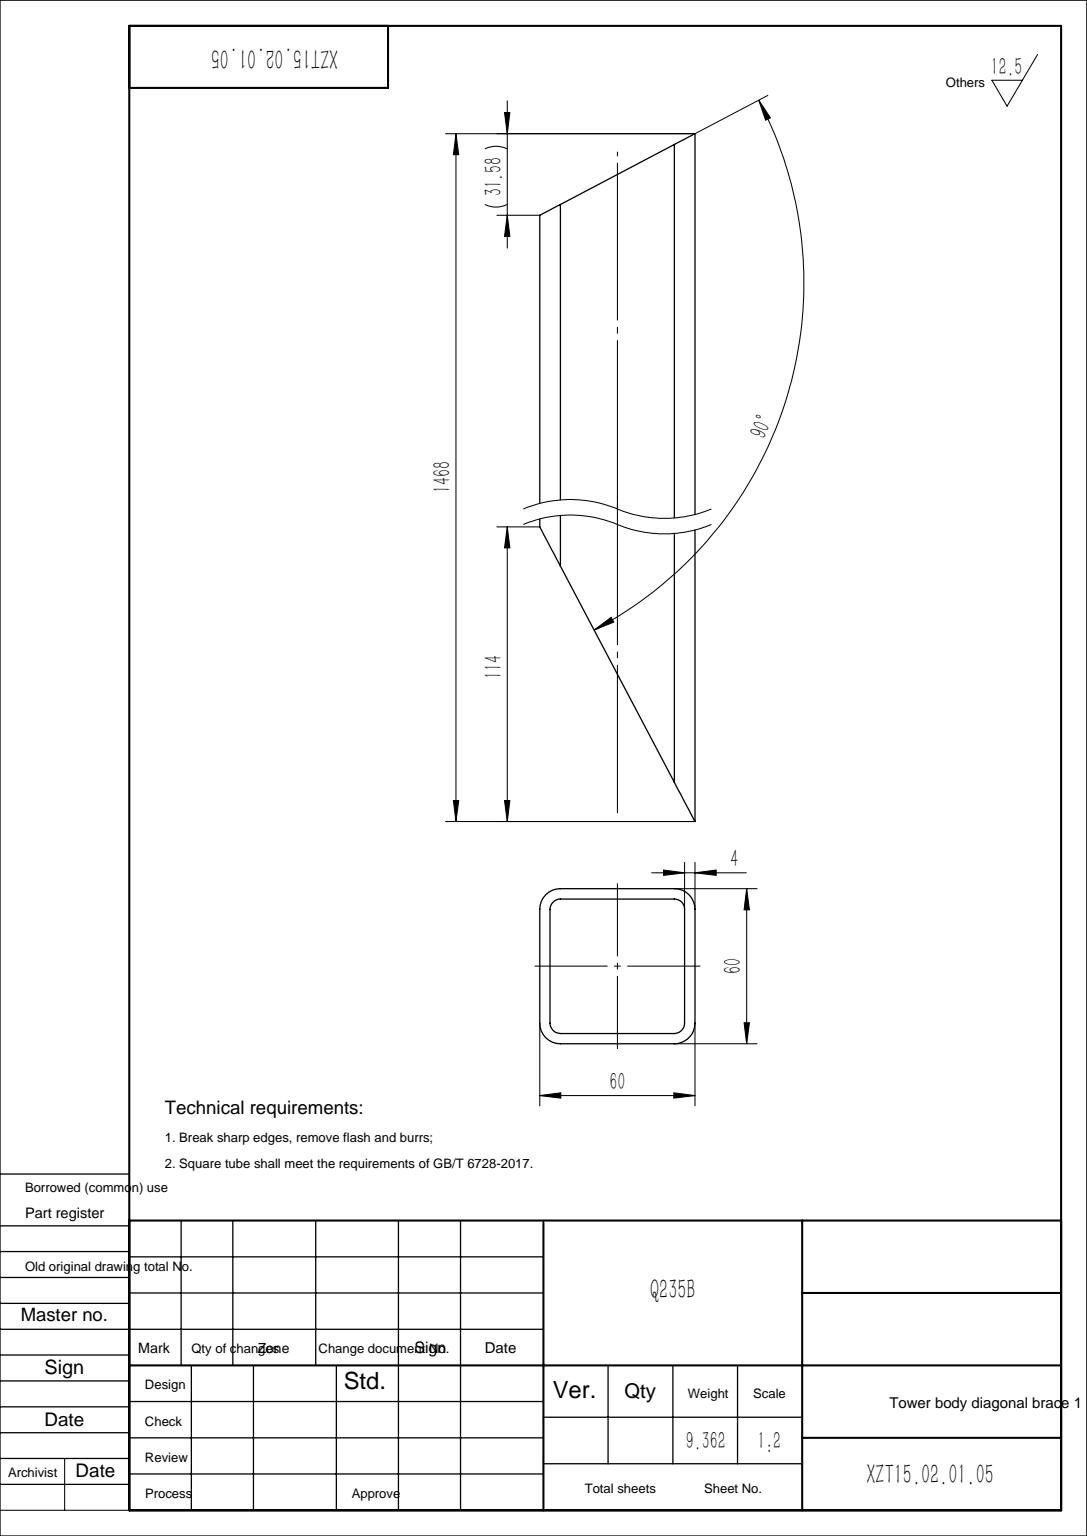
from build123d import *

# Parameters (mm, degrees)
GB_T_6728_2002_SQUARE_HOLLOW_SECTION_60_DEPTH = 1468
CUT_EXTRUDE1_DEPTH                            = 1470.531898259
CUT_EXTRUDE1_DEPTH_BACK                       = 1470.531898259


with BuildPart() as part:
    # Sketch1 → GB/T 6728-2002 square hollow section 60×60×4(1) (new body)
    with BuildSketch(Plane(origin=(0, 0, 0), x_dir=(-1, 0, 0), z_dir=(0, 1, 0))):
        with BuildLine():
            Line((-22, -30), (22, -30))
            ThreePointArc((22, -30), (27.656854249, -27.656854249), (30, -22))
            Line((30, -22), (30, 22))
            ThreePointArc((30, 22), (27.656854249, 27.656854249), (22, 30))
            Line((22, 30), (-22, 30))
            ThreePointArc((-22, 30), (-27.656854249, 27.656854249), (-30, 22))
            Line((-30, 22), (-30, -22))
            ThreePointArc((-30, -22), (-27.656854249, -27.656854249), (-22, -30))
        make_face()
        with BuildLine():
            Line((-22, -26), (22, -26))
            ThreePointArc((22, -26), (24.828427125, -24.828427125), (26, -22))
            Line((26, -22), (26, 22))
            ThreePointArc((26, 22), (24.828427125, 24.828427125), (22, 26))
            Line((22, 26), (-22, 26))
            ThreePointArc((-22, 26), (-24.828427125, 24.828427125), (-26, 22))
            Line((-26, 22), (-26, -22))
            ThreePointArc((-26, -22), (-24.828427125, -24.828427125), (-22, -26))
        make_face(mode=Mode.SUBTRACT)
    extrude(amount=GB_T_6728_2002_SQUARE_HOLLOW_SECTION_60_DEPTH)

    # Sketch2 → Cut-Extrude1 (cut, two sides: drawn at the far end of the back side and taken through both)
    with BuildSketch(Plane.XY.offset(30).offset(-CUT_EXTRUDE1_DEPTH_BACK)):
        Polygon((-30, 0), (-30, 114), (30, 0), align=None)
        Polygon((-30, 1436.421052632), (30, 1468), (-30, 1468), align=None)
    extrude(amount=CUT_EXTRUDE1_DEPTH + CUT_EXTRUDE1_DEPTH_BACK, mode=Mode.SUBTRACT)


solid = part.part
